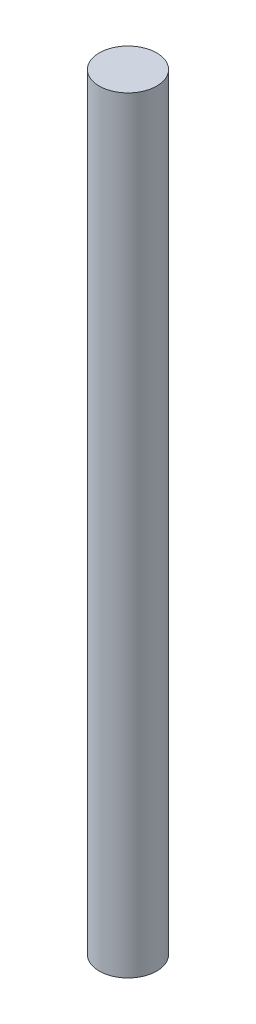
from build123d import *

# Parameters (mm, degrees)
SKETCH1_R           = 90
BOSS_EXTRUDE1_DEPTH = 2400


with BuildPart() as part:
    # Sketch1 → Boss-Extrude1 (new body)
    with BuildSketch(Plane(origin=(0, 0, 0), x_dir=(1, 0, 0), z_dir=(0, 1, 0))):
        with Locations(Location((0, 0, 0), (0, 0, 270))):
            Circle(SKETCH1_R)
    extrude(amount=BOSS_EXTRUDE1_DEPTH)


solid = part.part
